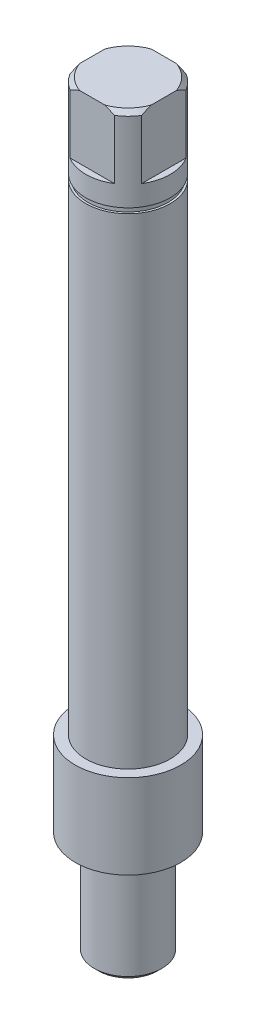
from build123d import *

# Parameters (mm, degrees)
CHAMFER1_SIZE           = 1
SKETCH3_W               = 5.79915747
SKETCH3_H               = 1.2
CUT_EXTRUDE2_DEPTH      = 181.865972477
CUT_EXTRUDE2_DEPTH_BACK = 181.865972477
SKETCH7_W               = 12.649467172
SKETCH7_H               = 42.427609508
CUT_EXTRUDE3_DEPTH      = 181.865972477
CUT_EXTRUDE3_DEPTH_BACK = 181.865972477
SKETCH8_W               = 5.603563882
SKETCH8_H               = 43.977481417


with BuildPart() as part:
    # Sketch1 → Revolve1 (revolve)
    with BuildSketch(Plane.XY, mode=Mode.PRIVATE) as revolve1_sk:
        Polygon((0, 180), (10, 180), (10, 45), (12.5, 45), (12.5, 25), (8, 25), (8, 0), (0, 0), align=None)
    revolve(revolve1_sk.sketch.rotate(Axis((0, 0, 0), (0, 1, 0)), 90), axis=Axis((0, 0, 0), (0, 1, 0)))

    # Chamfer1
    chamfer1_edges = [part.edges().sort_by_distance(p)[0] for p in [
        (0, 0, 8),
        (0, 180, 10),
    ]]
    chamfer(chamfer1_edges, length=CHAMFER1_SIZE)

    # Sketch3 → Cut-Revolve1 (revolve, cut)
    with BuildSketch(Plane.XY, mode=Mode.PRIVATE) as cut_revolve1_sk:
        with Locations((-12.399578735, 159.6)):
            Rectangle(SKETCH3_W, SKETCH3_H)
    revolve(cut_revolve1_sk.sketch.rotate(Axis((0, 180, 0), (0, -1, 0)), 270), axis=Axis((0, 180, 0), (0, -1, 0)), mode=Mode.SUBTRACT)

    # Sketch7 → Cut-Extrude2 (cut, two sides: drawn at the far end of the back side and taken through both)
    with BuildSketch(Plane.XY.offset(-CUT_EXTRUDE2_DEPTH_BACK)):
        with Locations((-14.824733586, 186.213804754)):
            Rectangle(SKETCH7_W, SKETCH7_H)
        with Locations((14.824733586, 186.213804754)):
            Rectangle(SKETCH7_W, SKETCH7_H)
    extrude(amount=CUT_EXTRUDE2_DEPTH + CUT_EXTRUDE2_DEPTH_BACK, mode=Mode.SUBTRACT)

    # Sketch8 → Cut-Extrude3 (cut, two sides: drawn at the far end of the back side and taken through both)
    with BuildSketch(Plane(origin=(0, 0, 0), x_dir=(0, 0, -1), z_dir=(1, 0, 0)).offset(-CUT_EXTRUDE3_DEPTH_BACK)):
        with Locations((-11.301781941, 186.988740709)):
            Rectangle(SKETCH8_W, SKETCH8_H)
        with Locations((11.301781941, 186.988740709)):
            Rectangle(SKETCH8_W, SKETCH8_H)
    extrude(amount=CUT_EXTRUDE3_DEPTH + CUT_EXTRUDE3_DEPTH_BACK, mode=Mode.SUBTRACT)


solid = part.part
